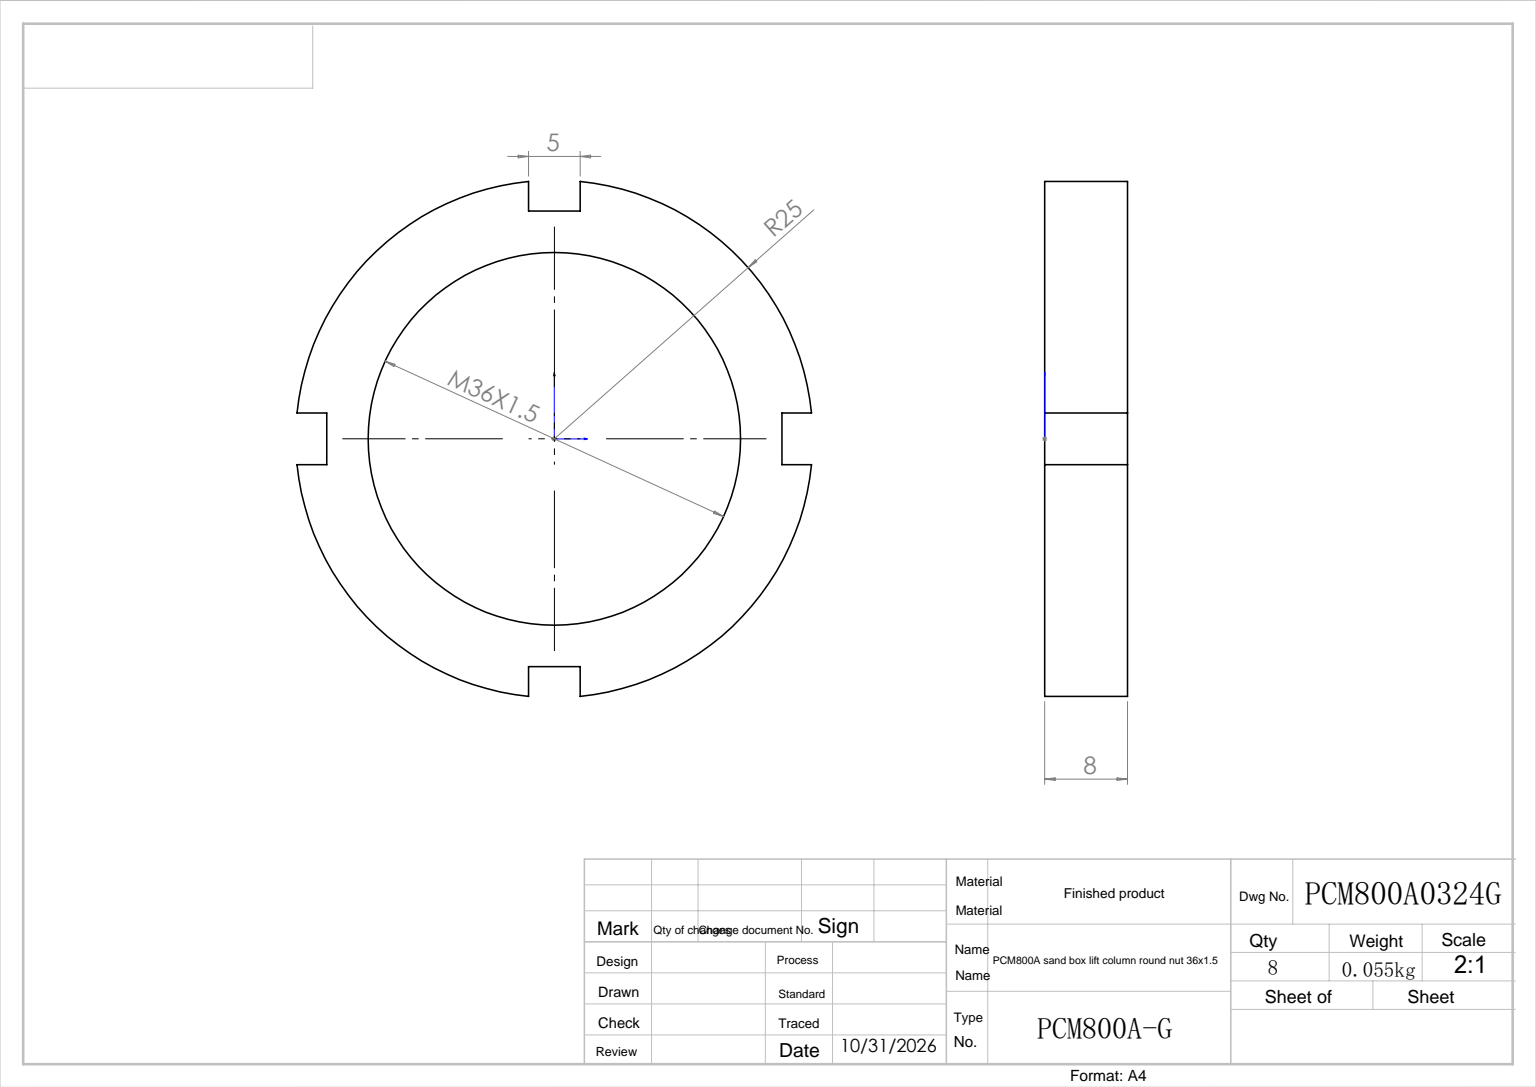
from build123d import *

# Parameters (mm, degrees)
SKETCH_1_R      = 18
EXTRUDE_1_DEPTH = 8


with BuildPart() as part:
    # 草图1 → 拉伸1 (new body)
    with BuildSketch(Plane.XY):
        with BuildLine():
            Line((-2.5, 24.871068248), (-2.5, 22))
            Line((-2.5, 22), (2.5, 22))
            Line((2.5, 22), (2.5, 24.871068248))
            ThreePointArc((2.5, 24.871068248), (17.675124268, 17.675124268), (24.871068248, 2.5))
            Line((24.871068248, 2.5), (22, 2.5))
            Line((22, 2.5), (22, -2.5))
            Line((22, -2.5), (24.871068248, -2.5))
            ThreePointArc((24.871068248, -2.5), (17.675124268, -17.675124268), (2.5, -24.871068248))
            Line((2.5, -24.871068248), (2.5, -22))
            Line((2.5, -22), (-2.5, -22))
            Line((-2.5, -22), (-2.5, -24.871068248))
            ThreePointArc((-2.5, -24.871068248), (-17.675124268, -17.675124268), (-24.871068248, -2.5))
            Line((-24.871068248, -2.5), (-22, -2.5))
            Line((-22, -2.5), (-22, 2.5))
            Line((-22, 2.5), (-24.871068248, 2.5))
            ThreePointArc((-24.871068248, 2.5), (-17.675124268, 17.675124268), (-2.5, 24.871068248))
        make_face()
        Circle(SKETCH_1_R, mode=Mode.SUBTRACT)
    extrude(amount=EXTRUDE_1_DEPTH)


solid = part.part
